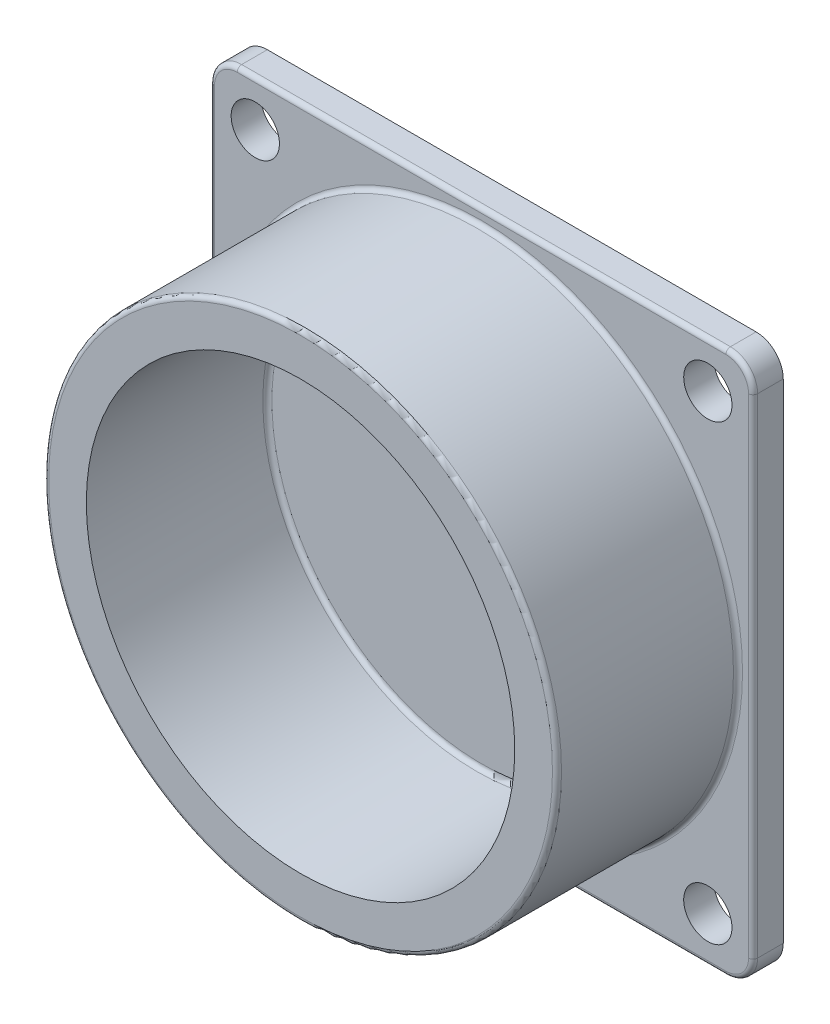
from build123d import *

# Parameters (mm, degrees)
SKETCH1_R           = 9
SKETCH1_R_2         = 4.5
BOSS_EXTRUDE1_DEPTH = 10
SKETCH2_R           = 85
BOSS_EXTRUDE2_DEPTH = 60
SKETCH3_R           = 71
CUT_EXTRUDE1_DEPTH  = 60
FILLET1_R           = 1.5
SCALE1_SCALE        = 0.5
SKETCH_1_R          = 2.25
EXTRUDE_1_DEPTH     = 5
SKETCH_2_R          = 4
CUT_EXTRUDE_1_DEPTH = 10


with BuildPart() as part:
    # Sketch1 → Boss-Extrude1 (new body)
    with BuildSketch(Plane.XY):
        with BuildLine():
            Line((-81, -90), (81, -90))
            ThreePointArc((81, -90), (87.363961031, -87.363961031), (90, -81))
            Line((90, -81), (90, 81))
            ThreePointArc((90, 81), (87.363961031, 87.363961031), (81, 90))
            Line((81, 90), (-81, 90))
            ThreePointArc((-81, 90), (-87.363961031, 87.363961031), (-90, 81))
            Line((-90, 81), (-90, -81))
            ThreePointArc((-90, -81), (-87.363961031, -87.363961031), (-81, -90))
        make_face()
        Circle(SKETCH1_R, mode=Mode.SUBTRACT)
        with Locations((70, 70)):
            Circle(SKETCH1_R_2, mode=Mode.SUBTRACT)
        with Locations(Location((-70, 70, 0), (0, 0, 180))):
            Circle(SKETCH1_R_2, mode=Mode.SUBTRACT)
        with Locations(Location((70, -70, 0), (0, 0, 180))):
            Circle(SKETCH1_R_2, mode=Mode.SUBTRACT)
        with Locations((-70, -70)):
            Circle(SKETCH1_R_2, mode=Mode.SUBTRACT)
    extrude(amount=BOSS_EXTRUDE1_DEPTH)

    # Sketch2 → Boss-Extrude2 (add)
    with BuildSketch(Plane.XY.offset(10)):
        with Locations(Location((0, 0, 0), (0, 0, 180))):
            Circle(SKETCH2_R)
    extrude(amount=BOSS_EXTRUDE2_DEPTH)

    # Sketch3 → Cut-Extrude1 (cut)
    with BuildSketch(Plane.XY.offset(70)):
        Circle(SKETCH3_R)
    extrude(amount=-CUT_EXTRUDE1_DEPTH, mode=Mode.SUBTRACT)

    # Fillet1
    fillet1_edges = [part.edges().sort_by_distance(p)[0] for p in [
        (87.363961031, 87.363961031, 10),
        (0, 90, 10),
        (-87.363961031, 87.363961031, 10),
        (-90, 0, 10),
        (-87.363961031, -87.363961031, 10),
        (0, -90, 10),
        (87.363961031, -87.363961031, 10),
        (85, 0, 10),
        (85, 0, 70),
        (-71, 0, 10),
        (90, 0, 10),
    ]]
    fillet(fillet1_edges, radius=FILLET1_R)


with BuildPart() as part_1:
    # Scale1: scaled about (0, 0, 0)
    add(part.part.scale(SCALE1_SCALE))

    # 草图1 → 凸台-拉伸1 (add)
    with BuildSketch(Plane(origin=(0, 0, 0), x_dir=(-1, 0, 0), z_dir=(0, 0, -1))):
        with Locations((35, -35)):
            Circle(SKETCH_1_R)
        with Locations((-35, -35)):
            Circle(SKETCH_1_R)
        with Locations((-35, 35)):
            Circle(SKETCH_1_R)
        with Locations((35, 35)):
            Circle(SKETCH_1_R)
    extrude(amount=-EXTRUDE_1_DEPTH)

    # 草图2 → 切除-拉伸1 (cut)
    with BuildSketch(Plane(origin=(0, 0, 0), x_dir=(-1, 0, 0), z_dir=(0, 0, -1))):
        with Locations((-37.5, 37.5)):
            Circle(SKETCH_2_R)
        with Locations(Location((-37.5, -37.5, 0), (0, 0, 180))):
            Circle(SKETCH_2_R)
        with Locations(Location((37.5, 37.5, 0), (0, 0, 180))):
            Circle(SKETCH_2_R)
        with Locations((37.5, -37.5)):
            Circle(SKETCH_2_R)
    extrude(amount=-CUT_EXTRUDE_1_DEPTH, mode=Mode.SUBTRACT)


solid = part_1.part
